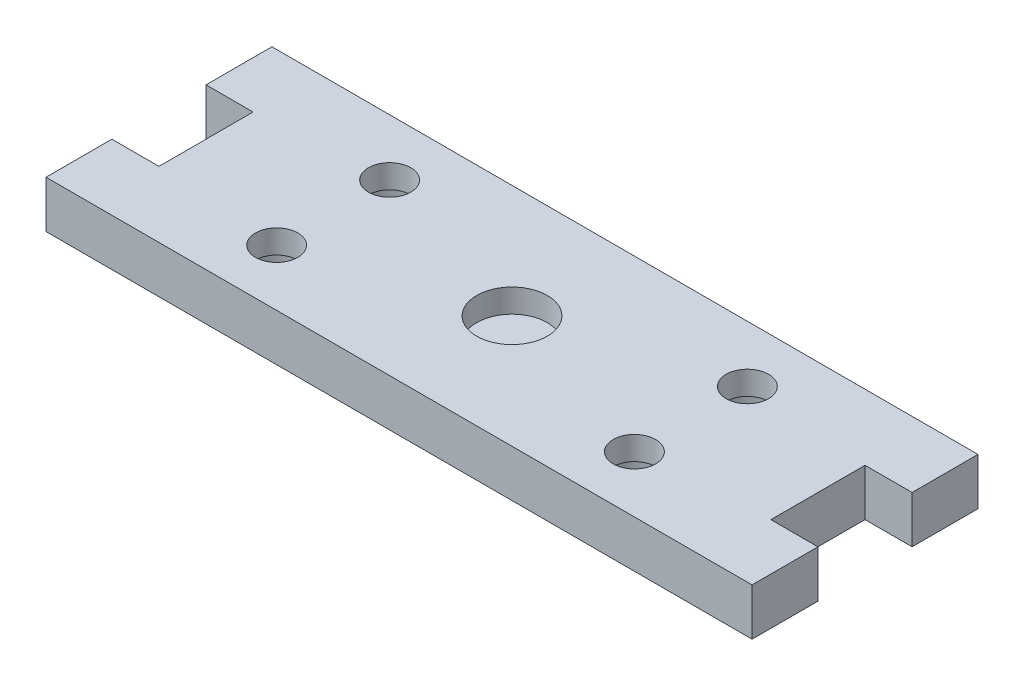
SolidWorks part; units mm, degrees
ref_plane "Front Plane" through (0, 0, 0) normal (0, 0, 1) x (1, 0, 0)
ref_plane "Top Plane" through (0, 0, 0) normal (0, 1, 0) x (1, 0, 0)
ref_plane "Right Plane" through (0, 0, 0) normal (1, 0, 0) x (0, 0, -1)
sketch "Sketch1" plane through (0, 0, 0) normal (0, 1, 0) x (1, 0, 0)
  line L1 (-75, 24) -> (75, 24)
  line L2 (-75, 24) -> (-75, -24)
  line L3 (-75, -24) -> (75, -24)
  line L4 (75, 24) -> (75, -24)
  line L5 (-75, 24) -> (75, -24) construction
  line L6 (-75, -24) -> (75, 24) construction
  point P0 (0, 0)
  dimension "D1" = 150
  dimension "D2" = 48
extrude "Boss-Extrude1" add sketch "Sketch1" along normal blind 10
hole_wizard "CBORE for M8 Cheese Head Screw1" positions "Sketch3" profile "Sketch4" counterbore size "M8" standard "ISO"
sketch "Sketch3" plane through (0, 0, 0) normal (0, -1, 0) x (-1, 0, 0)
  line L0 (-38, -12) -> (38, -12) construction
  line L2 (0, -24) -> (0, 24) construction
  line L3 (75, -24) -> (-75, -24) construction
  line L4 (-75, 24) -> (75, 24) construction
  line L6 (-75, -24) -> (-75, 24) construction
  line L7 (-38, -12) -> (-38, 12) construction
  line L8 (-38, 12) -> (38, 12) construction
  line L9 (38, 12) -> (38, -12) construction
  point P0 (-38, -12)
  point P2 (38, -12)
  point P16 (0, -12)
  point P22 (-38, 12)
  point P24 (38, 12)
  point P34 (0, 0)
  dimension "D1" = 76
  dimension "D2" = 37
  dimension "D3" = 76
  dimension "D4" = 24
  dimension "D5" = 12
  dimension "D6" = 12
  dimension "D7" = 38
sketch "Sketch4" plane through (38, 0, 12) normal (1, 0, 0) x (0, 0, -1)
  line L0 (0, 0) -> (0, 12.7039)
  line L1 (0, 12.7039) -> (4.5, 10)
  line L2 (4.5, 10) -> (4.5, 5)
  line L3 (4.5, 5) -> (7.5, 5)
  line L5 (7.5, 5) -> (7.5, 0.025)
  line L6 (7.5, 0.025) -> (7.525, 0)
  line L7 (7.525, 0) -> (0, 0)
  line L8 (-7.5, 0.025) -> (-7.525, 0) construction
  line L10 (0, 12.7039) -> (-4.5, 10) construction
  line L11 (0, -6.35) -> (0, 107.95) construction
  dimension "Hole Dia." = 9
  dimension "Hole Depth" = 10
  dimension "C'Bore Dia." = 15
  dimension "C'Bore Depth" = 5
  dimension "Near C'Sink Dia." = 15.05
  dimension "Near C'Sink Angle" = 90
  dimension "Drill Angle" = 118
sketch "Sketch6" plane through (0, 10, 0) normal (0, 1, 0) x (1, 0, 0)
  circle A0 centre (0, 0) radius 7.5
  dimension "D1" = 15
extrude "Cut-Extrude2" cut sketch "Sketch6" against normal blind 5
sketch "Sketch7" plane through (0, 10, 0) normal (0, 1, 0) x (1, 0, 0)
  line L0 (75, -24) -> (75, 24) construction
  line L1 (65, -10) -> (85, -10)
  line L2 (65, -10) -> (65, 10)
  line L3 (65, 10) -> (85, 10)
  line L4 (85, -10) -> (85, 10)
  line L5 (65, -10) -> (85, 10) construction
  line L6 (65, 10) -> (85, -10) construction
  line L7 (0, -24) -> (0, 24) construction
  line L8 (-75, -24) -> (75, -24) construction
  line L9 (75, 24) -> (-75, 24) construction
  line L10 (-65, 10) -> (-85, -10) construction
  line L11 (-65, -10) -> (-85, 10) construction
  line L12 (-85, -10) -> (-85, 10)
  line L13 (-65, 10) -> (-85, 10)
  line L14 (-65, -10) -> (-65, 10)
  line L15 (-65, -10) -> (-85, -10)
  point P0 (75, 0)
  point P17 (-75, 0)
  dimension "D1" = 20
  dimension "D2" = 20
extrude "Cut-Extrude3" cut sketch "Sketch7" against normal through all
